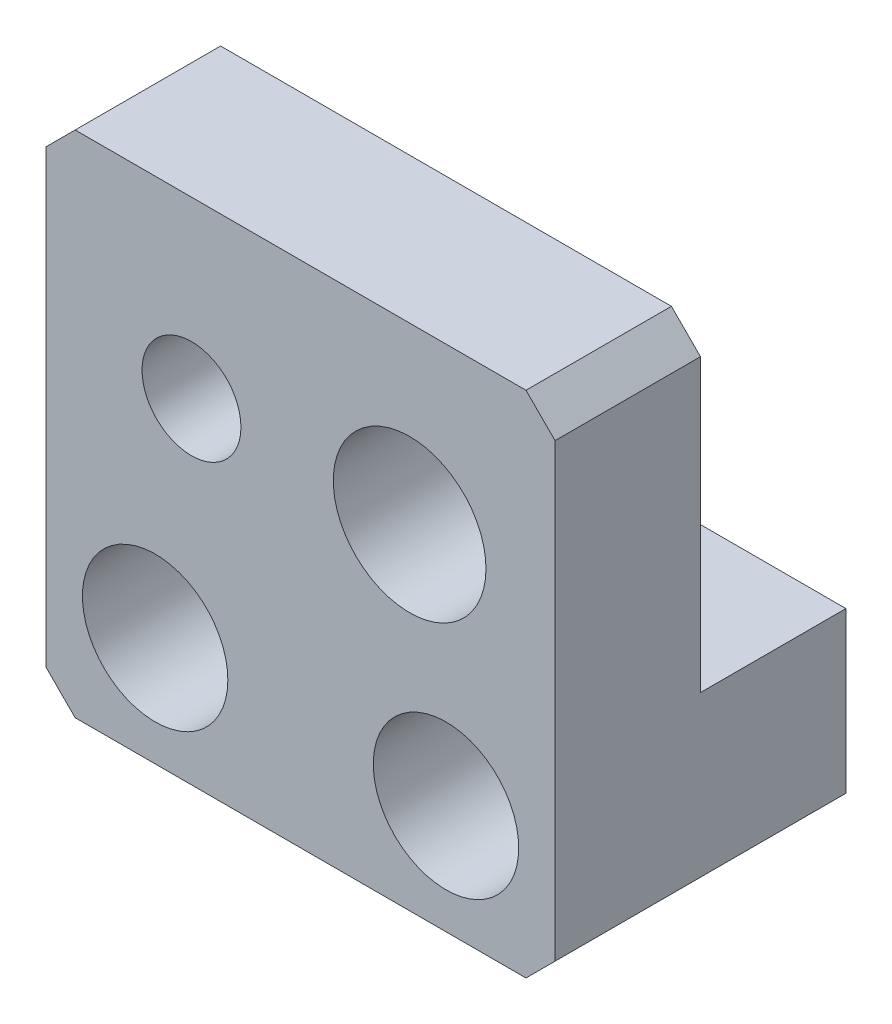
SolidWorks part; units mm, degrees
ref_plane "前视基准面" through (0, 0, 0) normal (0, 0, 1) x (1, 0, 0)
ref_plane "上视基准面" through (0, 0, 0) normal (0, 1, 0) x (1, 0, 0)
ref_plane "右视基准面" through (0, 0, 0) normal (1, 0, 0) x (0, 0, -1)
sketch "草图1" plane through (0, 0, 0) normal (0, 0, 1) x (1, 0, 0)
  line L9 (-17.5, -17.5) -> (17.5, -17.5)
  line L10 (-17.5, -17.5) -> (-17.5, 17.5)
  line L11 (-17.5, 17.5) -> (17.5, 17.5)
  line L12 (17.5, -17.5) -> (17.5, 17.5)
  line L13 (-17.5, -17.5) -> (17.5, 17.5) construction
  line L14 (-17.5, 17.5) -> (17.5, -17.5) construction
  point P0 (0, 0)
  dimension "D1" = 35
  dimension "D2" = 35
extrude "凸台-拉伸1" add sketch "草图1" along normal blind 20
chamfer "倒角1" distance 2 angle 45 4 edges at (17.5, -17.5, 10) (-17.5, -17.5, 10) (-17.5, 17.5, 10) (17.5, 17.5, 10)
sketch "草图4" plane through (0, 0, 20) normal (0, 0, 1) x (1, 0, 0)
  point P0 (7.5, 5.5)
hole_wizard "M12x1.25 螺纹孔1" positions "草图4" profile "草图3" tap size "M12x1.25" standard "GB" end condition through all
sketch "草图3" plane through (7.5, 5.5, 20) normal (1, 0, 0) x (0, -1, 0)
  line L0 (0, 0) -> (0, 20)
  line L1 (0, 20) -> (5.25, 20)
  line L2 (5.25, 20) -> (5.25, 0)
  line L5 (5.25, 0) -> (0, 0)
  line L11 (0, -6.35) -> (0, 107.95) construction
  dimension "通孔螺纹孔钻头直径" = 10.5
  dimension "通孔螺纹孔钻头深度" = 20
cosmetic thread "孔螺纹线1" parameters "D2"=12
sketch "草图7" plane through (0, 0, 20) normal (0, 0, 1) x (1, 0, 0)
  line L0 (0, 0) -> (0, 29.1951) construction
  line L2 (15.5, 17.5) -> (-15.5, 17.5) construction
  circle A0 centre (7.5, 5.5) radius 5.25 construction
  point P0 (-7.5, 5.5)
  dimension "D1" = 15
  dimension "D2" = 12
hole_wizard "M8 螺纹孔1" positions "草图7" profile "草图6" tap size "M8" standard "GB" end condition through all
sketch "草图6" plane through (-7.5, 5.5, 20) normal (1, 0, 0) x (0, -1, 0)
  line L0 (0, 0) -> (0, 20)
  line L1 (0, 20) -> (3.4, 20)
  line L2 (3.4, 20) -> (3.4, 0)
  line L5 (3.4, 0) -> (0, 0)
  line L11 (0, -6.35) -> (0, 107.95) construction
  dimension "通孔螺纹孔钻头直径" = 6.8
  dimension "通孔螺纹孔钻头深度" = 20
cosmetic thread "孔螺纹线2" parameters "D2"=8
sketch "草图10" plane through (0, 0, 20) normal (0, 0, 1) x (1, 0, 0)
  line L0 (0, 0) -> (0, 21.8687) construction
  line L2 (-15.5, -17.5) -> (15.5, -17.5) construction
  point P0 (-10, -10)
  point P2 (10, -10)
  dimension "D1" = 20
  dimension "D2" = 7.5
hole_wizard "M5 六角圆柱头螺钉的柱形沉头孔1" positions "草图10" profile "草图9" counterbore size "M5" standard "GB" end condition through all
sketch "草图9" plane through (-10, -10, 20) normal (1, 0, 0) x (0, -1, 0)
  line L0 (0, 0) -> (0, 20)
  line L1 (0, 20) -> (2.75, 20)
  line L3 (2.75, 20) -> (2.75, 12)
  line L4 (2.75, 12) -> (5, 12)
  line L5 (5, 12) -> (5, 0)
  line L7 (5, 0) -> (0, 0)
  line L11 (0, -6.35) -> (0, 107.95) construction
  dimension "通孔孔直径" = 5.5
  dimension "通孔孔深度" = 20
  dimension "柱形沉头孔直径" = 10
  dimension "柱形沉头孔深度" = 12
sketch "草图11" plane through (17.5, 0, 0) normal (1, 0, 0) x (0, 0, -1)
  line L1 (0, 17.5) -> (-10, 17.5)
  line L2 (0, 17.5) -> (0, -4.5)
  line L3 (0, -4.5) -> (-10, -4.5)
  line L4 (-10, 17.5) -> (-10, -4.5)
  dimension "D1" = 10
  dimension "D2" = 13
extrude "切除-拉伸1" cut sketch "草图11" against normal through all
